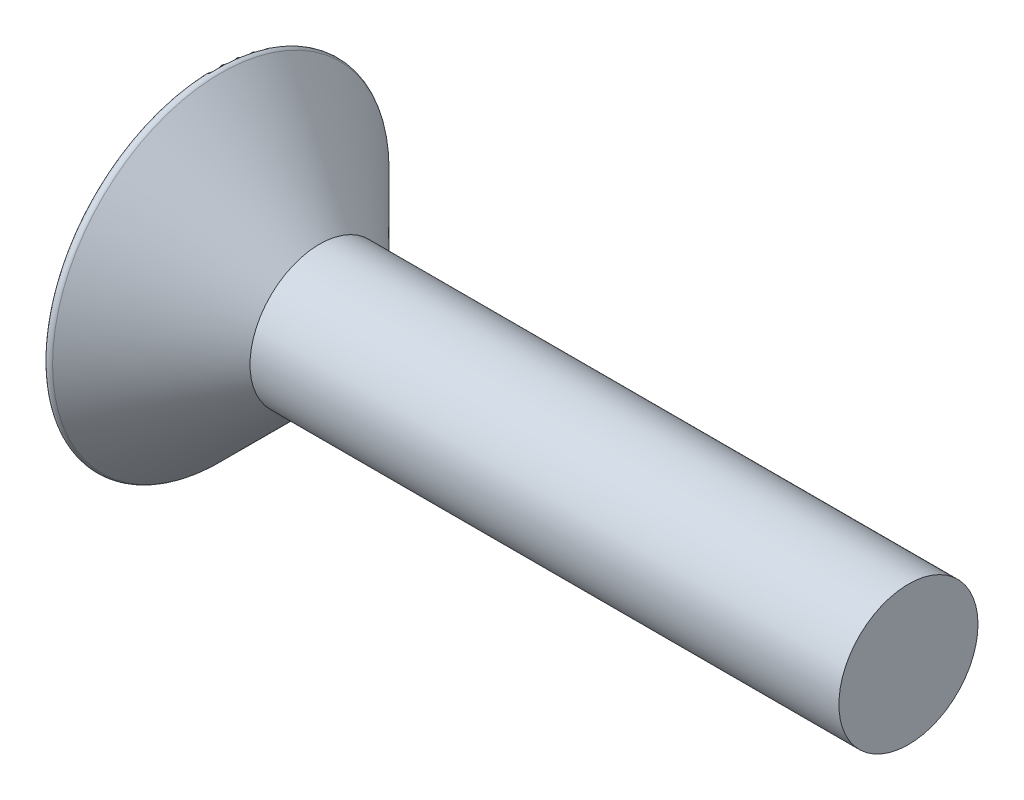
SolidWorks part; units mm, degrees
ref_plane "Front" through (0, 0, 0) normal (0, 0, 1) x (1, 0, 0)
ref_plane "Top" through (0, 0, 0) normal (0, 1, 0) x (1, 0, 0)
ref_plane "Right" through (0, 0, 0) normal (1, 0, 0) x (0, 0, -1)
other "Configuration Table"
ref_plane "Plane1" through (4.6, 0, 0) normal (1, 0, 0) x (0, 0, -1)
sketch "Sketch1" plane through (4.6, 0, 0) normal (1, 0, 0) x (0, 0, -1)
  circle A0 centre (0, 0) radius 3
extrude "BaseHead" add sketch "Sketch1" against normal blind 4.6 draft 45 draft outward yes
sketch "Sketch2" plane through (4.6, 0, 0) normal (1, 0, 0) x (0, 0, -1)
  circle A1 centre (0, 0) radius 3
extrude "BaseBody" add sketch "Sketch2" along normal blind 30
cosmetic thread "ThreadCosmetic1" [suppressed] parameters "bb"=23.4, "THD_MINOR"=5
sketch "Sketch7" plane through (0, 0, 0) normal (0, 0, 1) x (1, 0, 0)
  line L0 (30, 6) -> (30, -6)
  line L1 (34.6, -3) -> (34.6, 3) construction
  line L2 (34.6, 3) -> (4.6, 3) construction
  line L3 (4.6, -3) -> (34.6, -3) construction
extrude "Cut-Extrude3" cut sketch "Sketch7" against normal through all and the other way through all
sketch "Sketch8" plane through (0, 0, 0) normal (0, 0, 1) x (1, 0, 0)
  line L0 (0, 7.6) -> (4.6, 3)
  line L2 (6.3071, 2.7071) -> (6.6, 3)
  line L3 (6.6, 3) -> (6.6, 7.6)
  line L4 (6.6, 7.6) -> (0, 7.6)
  line L5 (30, 3) -> (4.6, 3) construction
  line L6 (0, 0) -> (8.9995, 0) construction
  line L7 (4.6, 3) -> (4.6, -3) construction
  arc A0 (4.6, 3) -> (6.3071, 2.7071) centre (5.6607, 4.0607) ccw
  dimension "r" = 1.5
  dimension "D1" = 45
  dimension "a" = 2
sketch "Sketch4" plane through (0, 0, 0) normal (1, 0, 0) x (0, 0, -1)
  line L1 (2.396, 0) -> (1.198, 2.075)
  line L2 (1.198, 2.075) -> (-1.198, 2.075)
  line L3 (-1.198, 2.075) -> (-2.396, 0)
  line L4 (-2.396, 0) -> (-1.198, -2.075)
  line L5 (-1.198, -2.075) -> (1.198, -2.075)
  line L6 (1.198, -2.075) -> (2.396, 0)
  circle A0 centre (0, 0) radius 2.075 construction
  dimension "B" = 4.15
extrude "Socket" cut sketch "Sketch4" along normal blind 2
sketch "Sketch5" plane through (2, 0, 0) normal (-1, 0, 0) x (0, 0, 1)
  line L0 (-1.198, 2.075) -> (1.198, 2.075) construction
  line L1 (1.198, 2.075) -> (2.396, 0) construction
  line L2 (2.396, 0) -> (1.198, -2.075) construction
  line L3 (1.198, -2.075) -> (-1.198, -2.075) construction
  line L4 (-2.396, 0) -> (-1.198, 2.075) construction
  line L5 (-1.198, -2.075) -> (-2.396, 0) construction
  line L6 (-1.198, 2.075) -> (1.198, 2.075)
  line L7 (1.198, 2.075) -> (2.396, 0)
  line L8 (2.396, 0) -> (1.198, -2.075)
  line L9 (1.198, -2.075) -> (-1.198, -2.075)
  line L10 (-2.396, 0) -> (-1.198, 2.075)
  line L11 (-1.198, -2.075) -> (-2.396, 0)
extrude "Cut-Extrude2" cut sketch "Sketch5" against normal blind 5 draft 60
sketch "Sketch6" plane through (-30.7487, 13.2487, 0) normal (0, 0, 1) x (0, -1, 0)
  line L0 (13.2487, 89.8637) -> (13.2487, 24.8312) construction
  line L1 (10.6609, 35.7609) -> (10.2487, 35.3487)
  line L2 (-7.1919, 35.3487) -> (-7.1919, 22.7487)
  line L3 (-7.1919, 22.7487) -> (10.2487, 22.7487)
  line L4 (10.7487, 35.973) -> (10.7487, 21.4009)
  line L5 (16.2487, 60.7487) -> (10.2487, 60.7487) construction
  line L6 (10.2487, 22.7487) -> (10.7487, 21.4009)
  line L8 (10.2487, 35.3487) -> (-7.1919, 35.3487)
  arc A0 (10.7487, 35.973) -> (10.6609, 35.7609) centre (10.4487, 35.973) cw
  dimension "D3" = 0.3
  dimension "d1" = 5
  dimension "b" = 38
  dimension "x" = 1.3478
fillet "HeadFillet" radius 0.2 1 edges at (0, 0, -7.6)
sketch "Sketch9" plane through (0, 0, 0) normal (0, 0, 1) x (1, 0, 0)
  line L0 (30, 2.567) -> (30.25, 3)
  line L1 (30.25, 3) -> (30.25, 3.5)
  line L2 (30.25, 3.5) -> (29.75, 3.5)
  line L3 (29.75, 3.5) -> (29.75, 3)
  line L4 (29.75, 3) -> (30, 2.567)
  line L5 (0, 0) -> (36.7555, 0) construction
  line L6 (30, -3) -> (30, 3) construction
revolve "Cut-Revolve10" [suppressed] cut sketch "Sketch9" angle 360 about L5
pattern_linear "LPattern10" [suppressed] count 7 spacing 0.6498 along (1, 0, 0)
equation "\"D1@Plane1\" = \"k@BaseHead\""
equation "\"D1@Sketch7\" = \"k@BaseHead\""
equation "\"D1@Sketch9\" = \"d@Sketch2\""
equation "\"D2@Sketch9\" =  ( \"d@Sketch2\" - \"THD_MINOR@ThreadCosmetic1\" )  / 2"
equation "\"D3@LPattern10\" = \"D2@Sketch9\" * 1.2"
equation "\"D1@LPattern10\" = \"bb@ThreadCosmetic1\" / \"D3@LPattern10\" "
